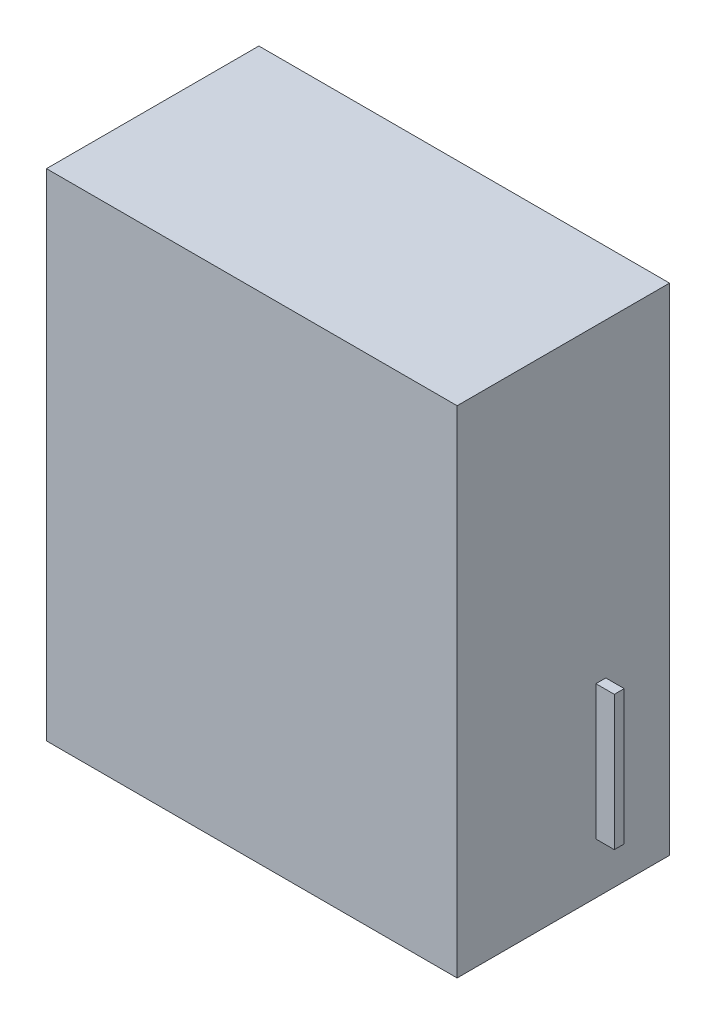
SolidWorks part; units mm, degrees
ref_plane "前视基准面" through (0, 0, 0) normal (0, 0, 1) x (1, 0, 0)
ref_plane "上视基准面" through (0, 0, 0) normal (0, 1, 0) x (1, 0, 0)
ref_plane "右视基准面" through (0, 0, 0) normal (1, 0, 0) x (0, 0, -1)
sketch "草图1" plane through (0, 0, 0) normal (0, 1, 0) x (1, 0, 0)
  line L1 (145, -75) -> (-145, -75)
  line L2 (145, -75) -> (145, 75)
  line L3 (145, 75) -> (-145, 75)
  line L4 (-145, -75) -> (-145, 75)
  line L5 (145, -75) -> (-145, 75) construction
  line L6 (145, 75) -> (-145, -75) construction
  point P0 (0, 0)
  dimension "D1" = 290
  dimension "D2" = 150
extrude "凸台-拉伸1" add sketch "草图1" along normal blind 350
sketch "草图2" plane through (0, 0, 0) normal (0, -1, 0) x (1, 0, 0)
  line L0 (0, 0) -> (0, 75) construction
  line L1 (-145, 75) -> (145, 75) construction
  circle A0 centre (-110, 63) radius 7
  circle A1 centre (110, 63) radius 7
  circle A2 centre (110, -67) radius 7
  circle A3 centre (-110, -67) radius 7
  dimension "D1" = 220
  dimension "D3" = 14
  dimension "D2" = 130
  dimension "D4" = 12
extrude "凸台-拉伸2" add sketch "草图2" along normal blind 5
sketch "草图3" plane through (-145, 0, 0) normal (-1, 0, 0) x (0, 0, 1)
  line L0 (0, -162.25) -> (0, 162.25) construction
  line L1 (72.5, 149) -> (-72.5, 149)
  line L2 (72.5, 149) -> (72.5, 172)
  line L3 (72.5, 172) -> (-72.5, 172)
  line L4 (-72.5, 149) -> (-72.5, 172)
  line L5 (72.5, 149) -> (-72.5, 172) construction
  line L6 (72.5, 172) -> (-72.5, 149) construction
  line L7 (-75, 0) -> (75, 0) construction
  point P0 (0, 160.5)
  dimension "D1" = 145
  dimension "D2" = 23
  dimension "D3" = 172
extrude "切除-拉伸1" cut sketch "草图3" against normal blind 1
sketch "草图4" plane through (-144, 0, 0) normal (-1, 0, 0) x (0, 0, 1)
  line L0 (-72.5, 160.5) -> (72.5, 160.5) construction
  line L1 (-46.5, 153) -> (-66.5, 153)
  line L2 (-46.5, 153) -> (-46.5, 168)
  line L3 (-46.5, 168) -> (-66.5, 168)
  line L4 (-66.5, 153) -> (-66.5, 168)
  line L5 (-46.5, 153) -> (-66.5, 168) construction
  line L6 (-46.5, 168) -> (-66.5, 153) construction
  line L7 (-72.5, 172) -> (-72.5, 149) construction
  line L8 (72.5, 149) -> (72.5, 172) construction
  line L9 (-72.5, 172) -> (-72.5, 149) construction
  point P0 (-56.5, 160.5)
  dimension "D1" = 20
  dimension "D2" = 15
  dimension "D3" = 6
extrude "凸台-拉伸3" add sketch "草图4" along normal blind 1.5
ref_plane "基准面1" through (0, 160.5, 0) normal (0, -1, 0) x (-1, 0, 0)
sketch "草图5" plane through (0, 160.5, 0) normal (0, -1, 0) x (-1, 0, 0)
  line L0 (145.5, 63.5) -> (149.5, 60.5)
  line L1 (145.5, 66.5) -> (145.5, 46.5) construction
  line L2 (145.5, 63.5) -> (145.5, 49.5)
  line L3 (145.5, 66.5) -> (144, 66.5) construction
  arc A0 (145.5, 49.5) -> (149.5, 60.5) centre (167.4305, 47.7525) cw
  dimension "D5" = 22
  dimension "D1" = 14
  dimension "D2" = 3
  dimension "D3" = 5
  dimension "D4" = 4
extrude "凸台-拉伸4" add sketch "草图5" along normal mid plane 9
sketch "草图6" plane through (145, 0, 0) normal (1, 0, 0) x (0, 0, -1)
  line L0 (82.5, 0) -> (-82.5, 0) construction
  line L1 (30, 36) -> (23, 36)
  line L2 (30, 36) -> (30, 131)
  line L3 (30, 131) -> (23, 131)
  line L4 (23, 36) -> (23, 131)
  line L5 (30, 36) -> (23, 131) construction
  line L6 (30, 131) -> (23, 36) construction
  line L7 (75, 350) -> (75, 0) construction
  point P0 (26.5, 83.5)
  dimension "D1" = 7
  dimension "D2" = 95
  dimension "D3" = 36
  dimension "D4" = 45
extrude "凸台-拉伸5" add sketch "草图6" along normal blind 13
